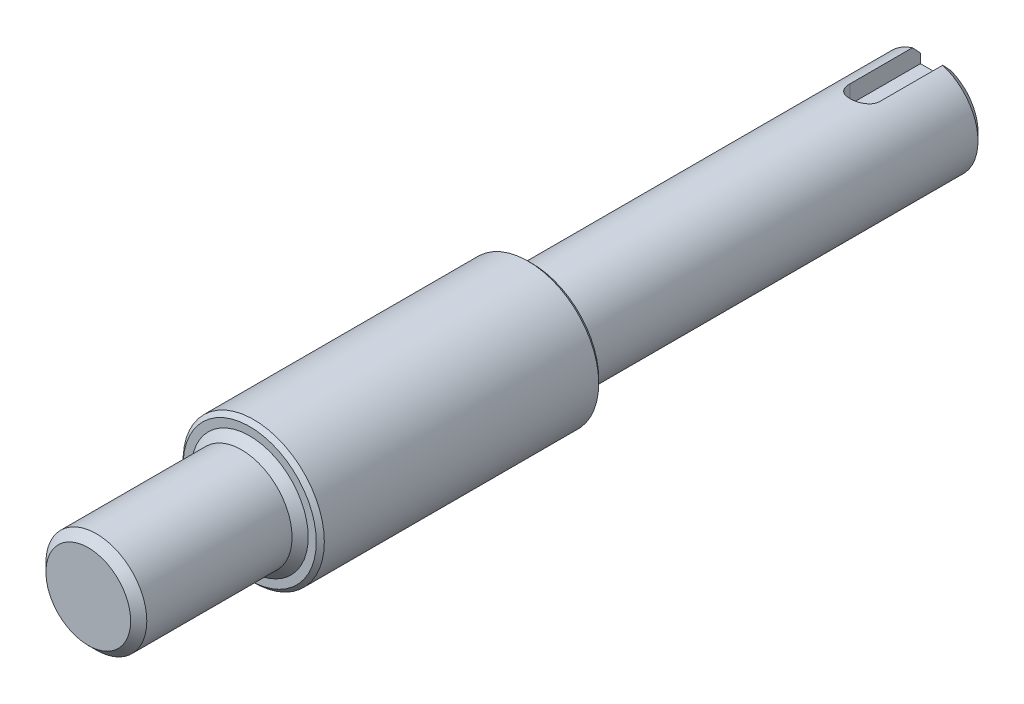
SolidWorks part; units mm, degrees
ref_plane "Front Plane" through (0, 0, 0) normal (0, 0, 1) x (1, 0, 0)
ref_plane "Top Plane" through (0, 0, 0) normal (0, 1, 0) x (1, 0, 0)
ref_plane "Right Plane" through (0, 0, 0) normal (1, 0, 0) x (0, 0, -1)
sketch "Sketch1" plane through (0, 0, 0) normal (0, 0, 1) x (1, 0, 0)
  circle A0 centre (0, 0) radius 25
  dimension "D1" = 50
extrude "Boss-Extrude1" add sketch "Sketch1" along normal blind 400 and the other way blind 20
chamfer "Chamfer1" distance 4 angle 45 2 edges at (25, 0, -20) (25, 0, 400)
ref_plane "Plane1" through (0, 25, 0) normal (0, 1, 0) x (1, 0, 0)
sketch "Sketch2" plane through (0, 25, 0) normal (0, 1, 0) x (1, 0, 0)
  line L0 (0, -236.8345) -> (0, -163.1655) construction
  line L2 (0, -200) -> (134.6003, -200) construction
  line L3 (7.5, -15) -> (7.5, 55)
  line L4 (7.5, 55) -> (-7.5, 55)
  line L5 (-7.5, -15) -> (-7.5, 55)
  line L6 (7.5, -15) -> (-7.5, 55) construction
  line L7 (7.5, 55) -> (-7.5, -15) construction
  line L8 (21, 20) -> (-21, 20) construction
  arc A0 (-7.5, -15) -> (7.5, -15) centre (0, -15) ccw
  point P3 (0, 20)
  dimension "D1" = 70
  dimension "D3" = 15
extrude "Cut-Extrude1" cut sketch "Sketch2" against normal blind 10
ref_plane "Plane2" through (0, 0, 250) normal (0, 0, 1) x (1, 0, 0)
sketch "Sketch3" plane through (0, 0, 250) normal (0, 0, 1) x (1, 0, 0)
  circle A0 centre (0, 0) radius 35
  dimension "D1" = 70
extrude "Boss-Extrude2" add sketch "Sketch3" along normal mid plane 140
chamfer "Chamfer2" distance 2 angle 45 2 edges at (35, 0, 180) (35, 0, 320)
chamfer "Chamfer3" distance 4 angle 45 2 edges at (25, 0, 180) (25, 0, 320)
